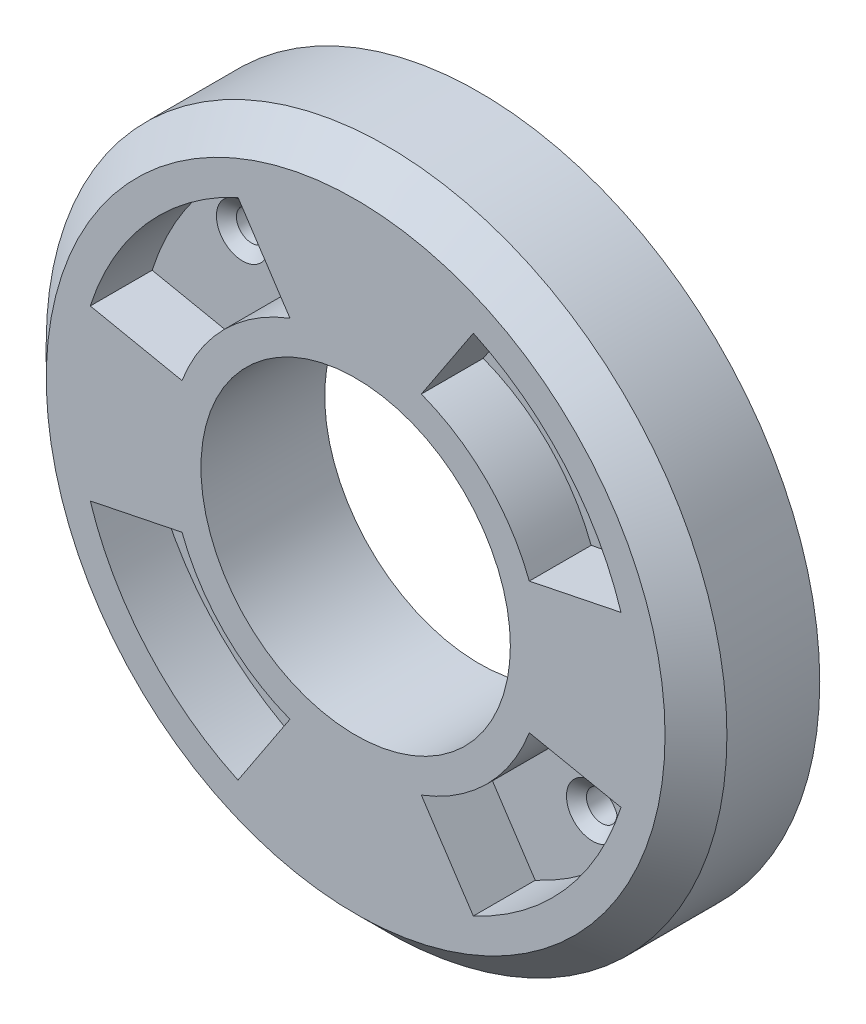
SolidWorks part; units mm, degrees
ref_plane "Front Plane" through (0, 0, 0) normal (0, 0, 1) x (1, 0, 0)
ref_plane "Top Plane" through (0, 0, 0) normal (0, 1, 0) x (1, 0, 0)
ref_plane "Right Plane" through (0, 0, 0) normal (1, 0, 0) x (0, 0, -1)
sketch "Sketch1" plane through (0, 0, 0) normal (0, 0, 1) x (1, 0, 0)
  circle A0 centre (0, 0) radius 55
  circle A1 centre (0, 0) radius 25
  dimension "D1" = 110
  dimension "D2" = 50
extrude "Boss-Extrude1" add sketch "Sketch1" along normal blind 20
sketch "Sketch2" plane through (0, 0, 20) normal (0, 0, 1) x (1, 0, 0)
  line L0 (0, 0) -> (0, 76.8274) construction
  line L1 (0, 0) -> (-67.4171, 0) construction
  line L2 (-10.6121, 28.0603) -> (-19.0171, 40.7842)
  line L3 (-28.0603, 10.6121) -> (-42.8824, 13.6419)
  line L4 (0, 0) -> (-21.2132, 21.2132) construction
  line L5 (28.0603, 10.6121) -> (42.8824, 13.6419)
  line L6 (10.6121, 28.0603) -> (19.0171, 40.7842)
  line L7 (10.6121, -28.0603) -> (19.0171, -40.7842)
  line L8 (28.0603, -10.6121) -> (42.8824, -13.6419)
  line L9 (-28.0603, -10.6121) -> (-42.8824, -13.6419)
  line L10 (-10.6121, -28.0603) -> (-19.0171, -40.7842)
  arc A0 (-19.0171, 40.7842) -> (-42.8824, 13.6419) centre (0, 0) ccw
  arc A1 (-10.6121, 28.0603) -> (-28.0603, 10.6121) centre (0, 0) ccw
  arc A2 (10.6121, 28.0603) -> (28.0603, 10.6121) centre (0, 0) cw
  arc A3 (19.0171, 40.7842) -> (42.8824, 13.6419) centre (0, 0) cw
  arc A4 (19.0171, -40.7842) -> (42.8824, -13.6419) centre (0, 0) ccw
  arc A5 (10.6121, -28.0603) -> (28.0603, -10.6121) centre (0, 0) ccw
  arc A6 (-10.6121, -28.0603) -> (-28.0603, -10.6121) centre (0, 0) cw
  arc A7 (-19.0171, -40.7842) -> (-42.8824, -13.6419) centre (0, 0) cw
  dimension "D1" = 90
  dimension "D2" = 60
  dimension "D3" = 45
  dimension "D4" = 45
extrude "Cut-Extrude1" cut sketch "Sketch2" against normal blind 10
chamfer "Chamfer1" distance 5 angle 45 1 edges at (55, 0, 20)
hole_wizard "CSK for #8 Flat Head Machine Screw (100)1" positions "3DSketch1" profile "Sketch3" countersink size "#8" standard "Ansi Inch" end condition through all
sketch3d "3DSketch1"
  line L0 (0, 0, 0) -> (0, 84.283, 0) construction
  line L2 (0, 0, 0) -> (-71.4787, 0, 0) construction
  line L4 (-28.2843, 26.4575, 10) -> (0, 0, 0) construction
  point P0 (-28.2843, 26.4575, 10)
  dimension "D1" = 45
  dimension "D2" = 40
sketch "Sketch3" plane through (-28.2843, 26.4575, 10) normal (1, 0, 0) x (0, -1, 0)
  line L0 (0, 0) -> (0, 10)
  line L1 (0, 10) -> (2.4574, 10)
  line L2 (2.4574, 10) -> (2.4574, 1.4759)
  line L3 (2.4574, 1.4759) -> (4.2164, 0)
  line L5 (4.2164, 0) -> (0, 0)
  line L6 (-2.4574, 1.4759) -> (-4.2164, 0) construction
  line L11 (0, -6.35) -> (0, 107.95) construction
  dimension "通孔孔直径" = 4.9149
  dimension "通孔孔深度" = 10
  dimension "近端锥形沉头孔直径" = 8.4328
  dimension "近端锥形沉头孔角度" = 100
mirror "Mirror1" about plane through (0, 0, 0) normal (1, 0, 0) of "CSK for #8 Flat Head Machine Screw (100)1"
mirror "Mirror2" about plane through (0, 0, 0) normal (0, 1, 0) of "Mirror1", "CSK for #8 Flat Head Machine Screw (100)1"
